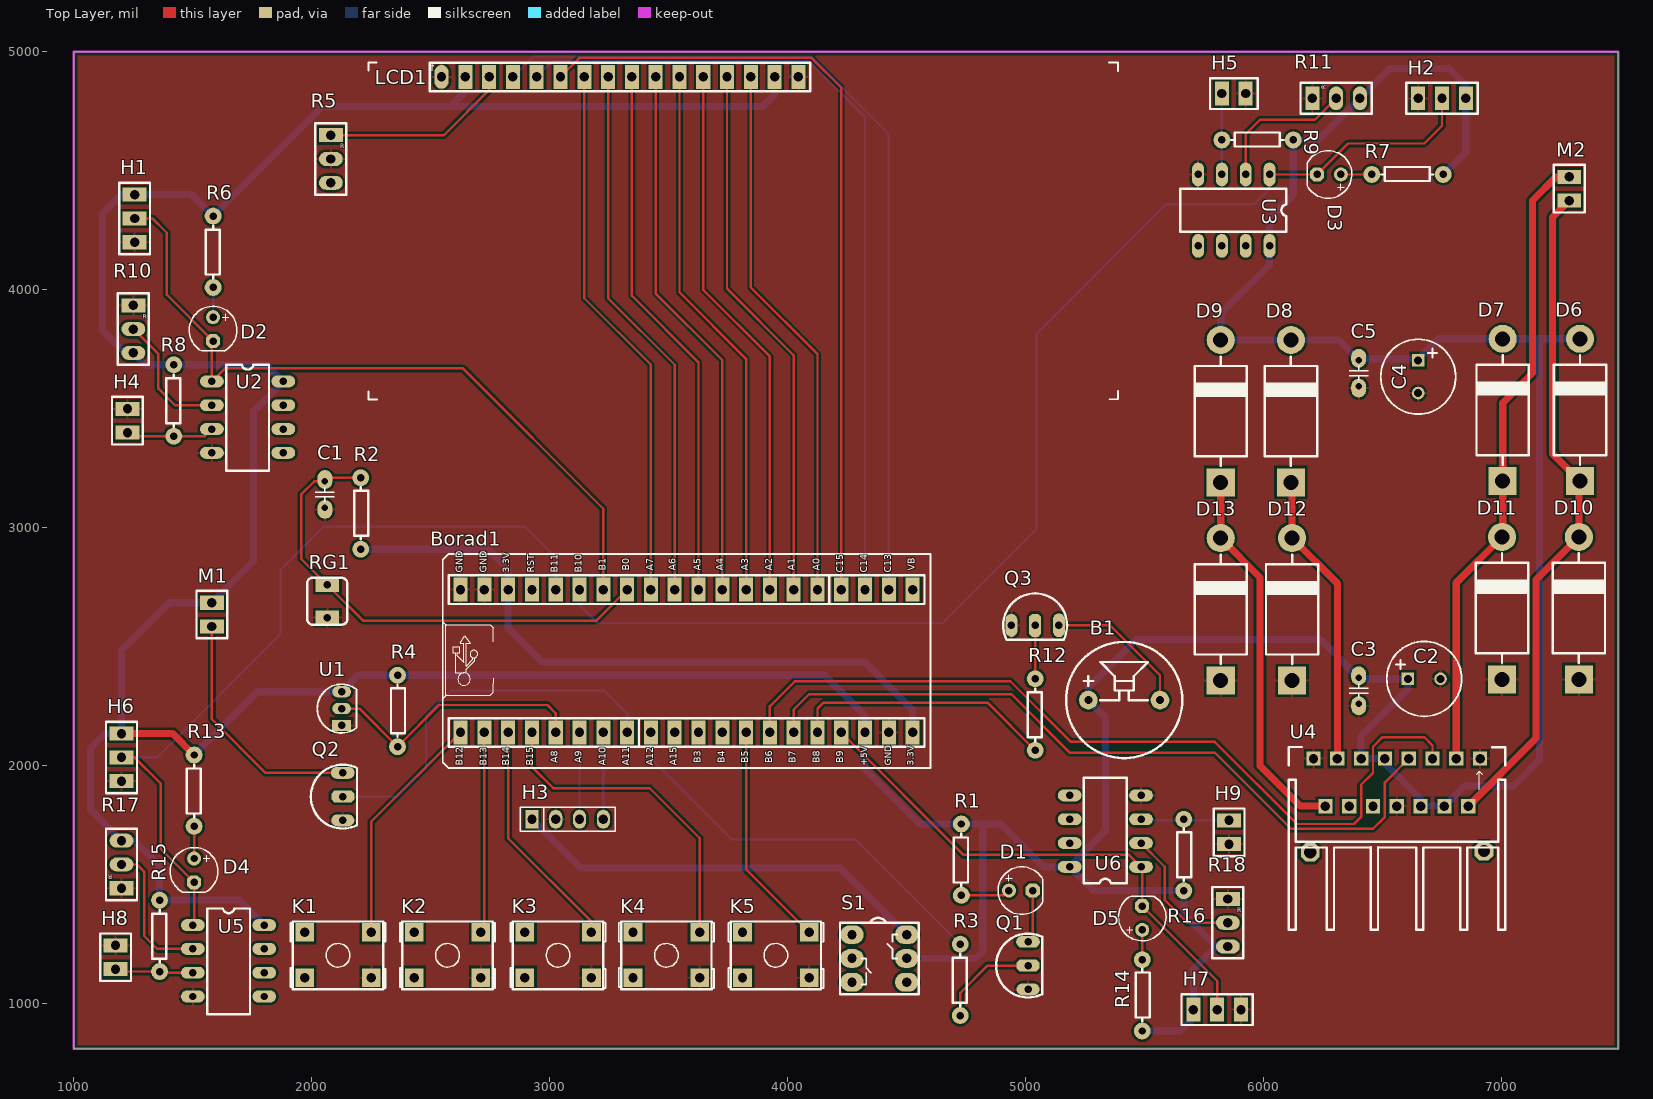
[diagram p0: Top Layer view]
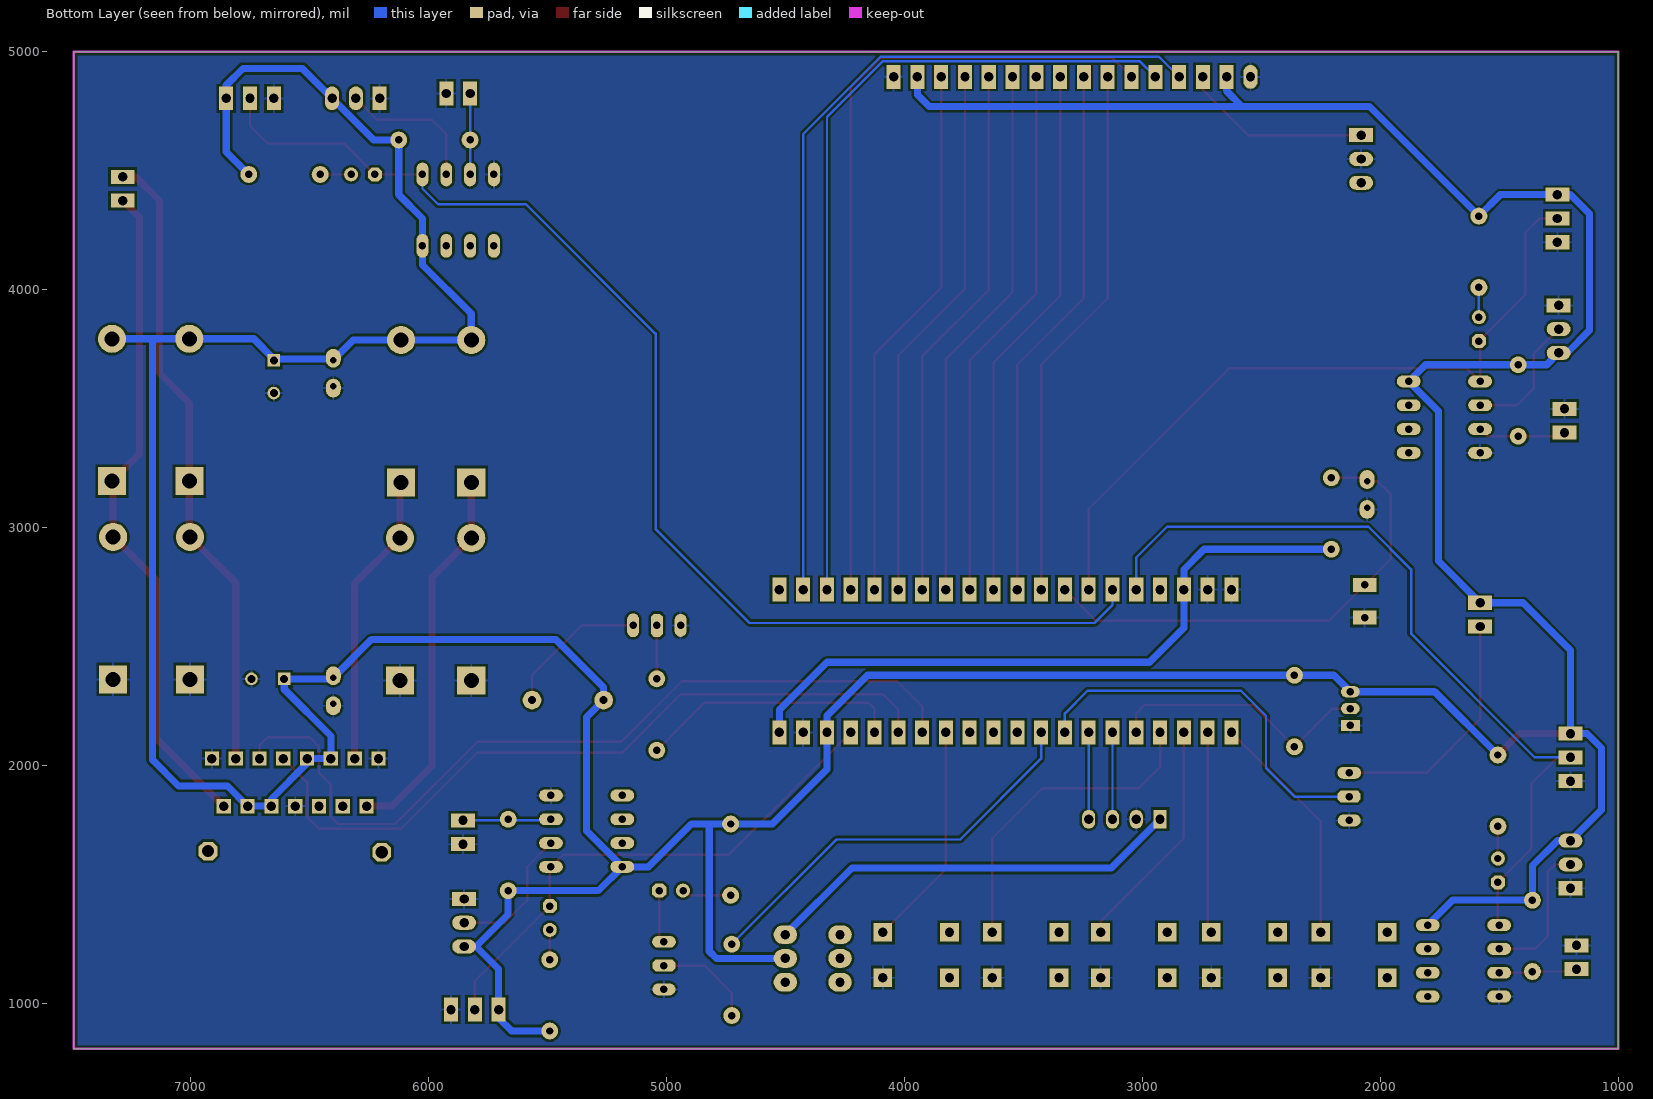
[diagram p1: Bottom Layer view, seen from below]
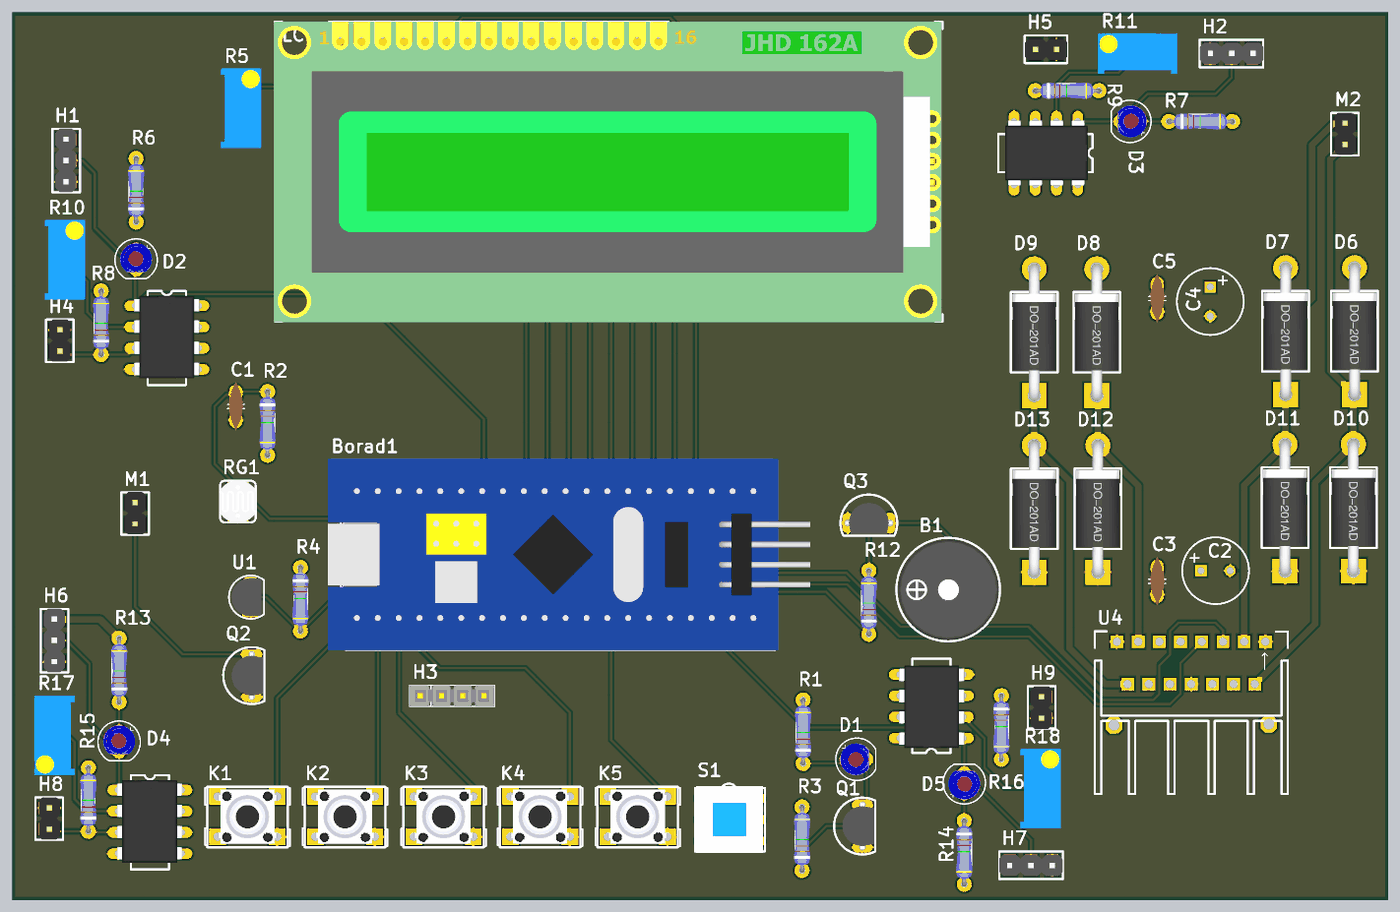
[diagram p2: 3D render of the assembled board from above, using the file's embedded part models]
# Altium PCB MISC82103.PcbDoc
Units mil, origin at the board's own origin, x right, y up, seen from the top; angles counter-clockwise.
Board outline 6490 x 4190 mil, 2 copper layers (Top Layer, Bottom Layer); 66 components, 56 nets, 252 pads, 0 vias.

## Layer stack, top to bottom (the 12.6 mil dielectric is the usual default, probably not edited)
Top Solder: solder mask 0.4, Solder Resist, Dk 3.5
Top Layer: signal copper 1.4
Dielectric 1: dielectric 12.6, FR-4, Dk 4.8
Bottom Layer: signal copper 1.4
Bottom Solder: solder mask 0.4, Solder Resist, Dk 3.5

## Board outline
1000,810 1000,5000 7490,5000 7490,810

## Design rules (kind name [scope] priority, off if disabled: settings)
Clearance [All] p1: gap=10
MinimumSolderMaskSliver [All] p1: minsoldermaskwidth=0
PolygonConnect [All] p1: connectstyle=Relief reliefconductorwidth=10 reliefentries=4 polygonreliefangle="90 Angle" airgapwidth=10
RoutingVias [All] p1: holewidth=28 width=50 viastyle="Through Hole" minholewidth=28 minwidth=50 maxholewidth=28 maxwidth=50
SilkToSilkClearance [All] p1: silktosilkclearance=0
SilkToSolderMaskClearance [IsPad] p1: minsilkscreentomaskgap=0 clearancetoexposedcopper=TRUE
SolderMaskExpansion [All] p1: expansion=4
Width [All] p1: maxlimit=50 minlimit=10 preferedwidth=10
27 further rules are at their usual default settings.

## Components (designator, comment, footprint, x,y, rotation, side; value= is the part's Value field where it differs from the comment)
B1 "Buzzer" BUZZER 5263.51,2275.91 r0 top
Borad1 "STM32F103C6T6_Borad" STM32F103C8T6_买的 2625,2140 r0 top
C1 "0.1uF" "CAP - 2.54mm" 2055,3140 r90 top
C2 "220uF" "CAPe - 3.5MM" 6675,2365 r0 top
C3 "0.1uF" "CAP - 2.54mm" 6400,2315 r90 top
C4 "220uF" "CAPe - 3.5MM" 6650,3635 r270 top
C5 "0.1uF" "CAP - 2.54mm" 6400,3650 r90 top
D1 "LED" LED-3MM 4980,1475 r180 top
D2 "LED" LED-3MM 1585,3835 r90 top
D3 "LED" LED-3MM 6275,4485 r0 top
D4 "LED" LED-3MM 1505,1560 r90 top
D5 "LED" LED-3MM 5490,1360 r270 top
D6 "1N4007" "DIODE - 15.24mm" 7330,3495 r270 top
D7 "1N4007" "DIODE - 15.24mm" 7005,3495 r270 top
D8 "1N4007" "DIODE - 15.24mm" 6115,3490 r270 top
D9 "1N4007" "DIODE - 15.24mm" 5820,3490 r270 top
D10 "1N4007" "DIODE - 15.24mm" 7325,2662.27 r270 top
D11 "1N4007" "DIODE - 15.24mm" 7002.36,2662.27 r270 top
D12 "1N4007" "DIODE - 15.24mm" 6120,2657.27 r270 top
D13 "1N4007" "DIODE - 15.24mm" 5820,2657.27 r270 top
H1 "CON3" CON3 1255,4300 r0 top
H2 "CON3" CON3 6750,4805 r270 top
H3 "Program download interface" CON4 3075,1775 r90 top
H4 "CON2" CON2 1225,3500 r0 top
H5 "CON2" CON2 5925,4825 r270 top
H6 "CON3" CON3 1200,2035 r0 top
H7 "CON3" CON3 5805,975 r90 top
H8 "CON2" CON2 1175,1245 r0 top
H9 "CON2" CON2 5855,1670 r180 top
K1 "Key" Buttom 2110,1205 r180 top
K2 "Key" Buttom 2570,1205 r180 top
K3 "Key" Buttom 3035,1205 r180 top
K4 "Key" Buttom 3490,1205 r180 top
K5 "Key" Buttom 3950,1205 r180 top
LCD1 "LCD1602" LCD1602 2545,4895 r0 top
M1 "FAN" CON2 1580,2685 r0 top
M2 "MOTTOR" CON2 7285,4475 r0 top
Q1 "NPN" "NPN & PNP" 5010,1160 r0 top
Q2 "NPN" "NPN & PNP" 2130,1870 r0 top
Q3 "NPN" "NPN & PNP" 5040,2590 r270 top
R1 "330R" Resistor-7.62mm 4730,1455 r90 top
R2 "10K" Resistor-7.62mm 2205,3210 r270 top
R3 "1K" Resistor-7.62mm 4725,950 r90 top
R4 "10K" Resistor-7.62mm 2360,2380 r270 top
R5 "10K" Res_Variable-DIP 2080,4650 r0 top
R6 "300R" Resistor-7.62mm 1585,4010 r90 top
R7 "300R" Resistor-7.62mm 6455,4485 r0 top
R8 "1M" Resistor-7.62mm 1420,3385 r90 top
R9 "1M" Resistor-7.62mm 5825,4630 r0 top
R10 "10K" Res_Variable-DIP 1250,3935 r0 top
R11 "10K" Res_Variable-DIP 6205,4805 r90 top
R12 "1K" Resistor-7.62mm 5040,2065 r90 top
R13 "300R" Resistor-7.62mm 1505,1745 r90 top
R14 "300R" Resistor-7.62mm 5490,1185 r270 top
R15 "1M" Resistor-7.62mm 1360,1135 r90 top
R16 "1M" Resistor-7.62mm 5665,1775 r270 top
R17 "10K" Res_Variable-DIP 1200,1485 r180 top
R18 "10K" Res_Variable-DIP 5850,1440 r0 top
RG1 "1M" RG 2065,2622.2 r180 top
S1 "Latching switch" Switch 4270,1190 r0 top
U1 "DS18B20" DS18B20 2125,2240 r90 top
U2 "LM358" DIP8 1780,3415 r0 top
U3 "LM358" DIP8 5825,4285 r270 top
U4 "L298N-DIP" L298N 6561,1931 r180 top
U5 "LM358" DIP8 1700,1130 r0 top
U6 "LM358" DIP8 5285,1775 r180 top

## Footprints (in the part's own frame and the unit in brackets; to place one, negate y for a bottom-side part, rotate by r counter-clockwise, add the part's x,y. Pads: shape width x height; smd on the part's side, far side on the other; paste and mask are expansions set on the pad)
Buttom [mm]
  rect 2x2 hole 1: 1(-3.556,2.438) 2(-3.556,-2.413) 3(3.556,-2.413) 4(3.556,2.438)
  silkscreen extent -5.08,-3.56 5.08,3.68, body extent -4.13,-3.22 4.13,3.28, height 5
BUZZER [mm] "蜂鸣器-DIP直插封装"
  round 2 hole 0.85: 1(0,0) 2(7.65,0)
  silkscreen extent -2.38,-6.2 10.02,6.2, body extent -2.14,-6.03 9.86,5.97, height 9.3
"CAP - 2.54mm" [mm] "2.54mm脚距陶瓷电容"
  oval 2x1.6 hole 0.7 copper offset -0.2,0: 1(-1.397,0)
  oval 2x1.6 hole 0.7 copper offset 0.2,0: 2(1.397,0)
  silkscreen extent -0.76,-1.02 0.76,1.02, body extent -2.9,-0.85 2.94,0.85, height 5.92
"CAPe - 3.5MM" [mm]
  rect 1.35x1.35 hole 0.85: 1(-1.75,0)
  round 1.35 hole 0.85: 2(1.75,0)
  silkscreen extent -4,-4 4,4
CON2 [mm]
  rect 2.54x1.5 hole 1: 1(0,0) 2(0,-2.54)
  silkscreen extent -1.65,-3.81 1.65,1.27, body extent -1.24,-3.78 1.3,1.3, height 8.54
CON3 [mm]
  rect 2.54x1.5 hole 1: 1(0,2.54) 2(0,0) 3(0,-2.54)
  silkscreen extent -1.65,-3.81 1.65,3.81, body extent -1.3,-3.78 1.24,3.84, height 8.54
CON4 [mm]
  rect 2x1.4 hole 1: 1(0,3.81)
  oval 2x1.4 hole 1: 2(0,1.27) 3(0,-1.27) 4(0,-3.81)
  silkscreen extent -1.27,-5.08 1.27,5.08, body extent -1.27,-5.08 1.27,5.08, height 8.89
"DIODE - 15.24mm" [mm] "间距15.24mm"
  rect 3x3 hole 1.6: 1(7.6,0)
  round 3 hole 1.6: 2(-7.6,0)
  silkscreen extent -5.84,-2.79 5.84,2.79, body extent -8.25,-2.6 8.25,2.6, height 5.25
DIP8 [mm]
  oval 2.54x1.27 hole 0.8: 1(-5.08,5.08) 2(-5.08,2.54) 3(-5.08,0) 4(-5.08,-2.54) 5(2.54,-2.54) 6(2.54,0) 7(2.54,2.54) 8(2.54,5.08)
  silkscreen extent -3.56,-4.44 1.02,6.85, body extent -5.21,-3.63 2.61,6.28, height 4.57
DS18B20 [mm]
  rect 1.2x2 hole 0.8: 1(-1.8,0)
  oval 1.2x2 hole 0.8: 2(0,0) 3(1.8,0)
  silkscreen extent -2.6,-1.6 2.6,2.6, body extent -2.3,-1.3 2.3,2.3, height 7.6
L298N [mil]
  oct 78.74x78.74 hole 51.18: 0(-365,290) 0(365,295)
  rect 60x60 hole 39.37: 1(-349,-99) 2(-299,101) 3(-249,-99) 4(-199,101) 5(-149,-99) 6(-99,101) 7(-49,-99) 8(1,101) 9(51,-99) 10(101,101) 11(151,-99) 12(201,101) 13(251,-99) 14(301,101) 15(351,-99)
  silkscreen extent -455,-148 455,620
LCD1602 [mm]
  oval 1.5x2.54 hole 1: 1(0,0)
  rect 1.5x2.54 hole 1: 2(2.54,0) 3(5.08,0) 4(7.62,0) 5(10.16,0) 6(12.7,0) 7(15.24,0) 8(17.78,0) 9(20.32,0) 10(22.86,0) 11(25.4,0) 12(27.94,0) 13(30.48,0) 14(33.02,0) 15(35.56,0) 16(38.1,0)
  silkscreen extent -7.8,-34.44 72.21,1.55, body extent -7.92,-34.46 72.08,1.54, height 10.6
LED-3MM [mm]
  oct 1.5x1.5 hole 0.8: 1(-1.27,0)
  round 1.5 hole 0.8: 2(1.27,0)
  silkscreen extent -2.35,-2.54 2.44,2.54, body extent -1.57,-1.9 1.93,1.93, height 5.5
"NPN & PNP" [mm]
  oct 2.45x1.27 hole 0.8: 1(0,0)
  oval 2.45x1.27 hole 0.8: 2(0,-2.54)
  oval 2.54x1.27 hole 0.8: 3(0,2.54)
  silkscreen extent -3.41,-3.41 1.52,3.41, body extent -2.41,-2.84 1.39,2.84, height 6.83
Res_Variable-DIP [mm]
  rect 2.54x1.5 hole 1: 1(0,0)
  oval 2.54x1.5 hole 1: 2(0,-2.54) 3(0,-5.08)
  silkscreen extent -1.65,-6.35 1.65,1.27, body extent -2.42,-7.38 2.41,2.15, height 11.55
Resistor-7.62mm [mm]
  round 1.8 hole 0.8: 1(0,0) 2(7.62,0)
  silkscreen extent 0.98,-0.7 6.58,0.8, body extent -0.25,-0.98 7.87,0.97, height 2.51
RG [mm] "光敏电阻"
  rect 2.54x1.5 hole 0.8: 1(0,0) 2(0,-3.5)
  silkscreen extent -2.13,-4.25 2.13,0.75, body extent -2.15,-4.28 2.15,0.77, height 2.2
STM32F103C8T6_买的 [mm] "买的小系统"
  rect 1.5x2.54 hole 1: 1(0,0) 2(2.54,0) 3(5.08,0) 4(7.62,0) 5(10.16,0) 6(12.7,0) 7(15.24,0) 8(17.78,0) 9(20.32,0) 10(22.86,0) 11(25.4,0) 12(27.94,0) 13(30.48,0) 14(33.02,0) 15(35.56,0) 16(38.1,0) 17(40.64,0) 18(43.18,0) 19(45.72,0) 20(48.26,0) 21(48.26,15.24) 22(45.72,15.24) 23(43.18,15.24) 24(40.64,15.24) 25(38.1,15.24) 26(35.56,15.24) 27(33.02,15.24) 28(30.48,15.24) 29(27.94,15.24) 30(25.4,15.24) 31(22.86,15.24) 32(20.32,15.24) 33(17.78,15.24) 34(15.24,15.24) 35(12.7,15.24) 36(10.16,15.24) 37(7.62,15.24) 38(5.08,15.24) 39(2.54,15.24) 40(0,15.24)
  silkscreen extent -1.91,-3.81 50.16,19.05, body extent -3.48,-3.85 54.32,19.15, height 11.4
Switch [mm]
  oval 2.5x2 hole 1: 1(0,2.54) 2(0,0) 3(0,-2.54) 4(5.842,-2.54) 5(5.842,0) 6(5.842,2.54)
  silkscreen extent -1.27,-3.81 7.11,4.32, body extent -1.12,-3.99 6.88,4.01, height 13.5

## Part data
Borad1: "Core board (purchased online)"
C1 C3 C5: library part CAP, "Non-polar capacitor"
C2 C4: library part CAP-E, "Polar capacitor"
D1: library part LED-RED
D2 D3 D4 D5: library part LED-GREEN
D6 D7 D8 D9 D10 D11 D12 D13: library part Diode, "Rectifier diode / single-direction diode"
H1 H2 H4 H5 H6 H7 H8 H9: "Pin header / terminal block / connector"
H3: library part CON4, "Pin header / terminal block / connector"
K1 K2 K3 K4 K5: "Push button"
M1: "Small fan"
M2: "DC motor"
Q1 Q2 Q3: "NPN transistor"
R1 R2 R3 R4 R6 R7 R8 R9 R12 R13 R14 R15 R16: library part Res, "Resistor"
R5 R10 R11 R17 R18: library part Res_Variable, "Adjustable resistor"
RG1: library part RG, "Photoresistor"
S1: library part Switch, "8*8 power switch / latching switch"
U1: "Temperature sensor"
U2 U3 U5 U6: "Dual operational amplifier"
U4: "Dual H-bridge driver IC"

## Nets (pads, with @x,y where several pads share a name; then routed paths per layer and width w, separated by ;. In a path a pad name is that pad's centre, name@x,y a point inside that pad or via, vN(x,y) a via of type N, cw(c..) or ccw(c..) an arc to the next point about the centre after c; other vN are vias at no path point)
+3.3V: Borad1.20 Borad1.38 R2.2 | length 2838.1
  Bottom Layer w30: R2.2 2740,2910 2825,2825 Borad1.38 2825,2580 2970,2435 4325,2435 4525,2235 Borad1.20
+5V: H3.1 S1.6 | length 1775.9
  Bottom Layer w30: H3.1 3130,1570 4220,1570 S1.6
BUZZER: Borad1.16 R12.1 | length 1108.2
  Top Layer w10: Borad1.16 4125,2240 4150,2265 4840,2265 R12.1
D0: Borad1.32 LCD1.7 | length 2271
  Top Layer w10: LCD1.7 3145,3965 3425,3685 Borad1.32
D1: Borad1.31 LCD1.8 | length 2271
  Top Layer w10: LCD1.8 3245,3965 3525,3685 Borad1.31
D2: Borad1.30 LCD1.9 | length 2271
  Top Layer w10: LCD1.9 3345,3975 3625,3695 Borad1.30
D3: Borad1.29 LCD1.10 | length 2271
  Top Layer w10: LCD1.10 3445,3985 3725,3705 Borad1.29
D4: Borad1.28 LCD1.11 | length 2271
  Top Layer w10: LCD1.11 3545,3990 3825,3710 Borad1.28
D5: Borad1.27 LCD1.12 | length 2271
  Top Layer w10: LCD1.12 3645,4000 3925,3720 Borad1.27
D6: Borad1.26 LCD1.13 | length 2271
  Top Layer w10: LCD1.13 3745,4005 4025,3725 Borad1.26
D7: Borad1.25 LCD1.14 | length 2271
  Top Layer w10: LCD1.14 3845,4010 4125,3730 Borad1.25
DS18B20: Borad1.5 R4.2 U1.2 | length 1133.3
  Top Layer w10: U1.2 2200,2240 R4.2 2535,2255 2990,2255 3025,2220 Borad1.5
EN: Borad1.24 LCD1.6 | length 3375.3
  Top Layer w10: LCD1.6 3045,4895.74 3124.26,4975 4100,4975 4225,4850 Borad1.24
ENA: B1.1 Borad1.18 C2.1 C3.2 C4.1 C5.2 D6.2 D7.2 D8.2 D9.2 H1.1 H2.1 H6.1 H7.1 LCD1.2 LCD1.15 M1.1 R1.2 R4.1 R6.2 R7.2 R8.2 R9.2 R10.3 R11.3 R13.2 R14.2 R15.2 R16.2 R17.3 R18.3 S1.5 U1.3 U2.8 U3.8 U4.4 U4.6 U4.9 U4.11 U5.8 U6.8 | length 24220
  Top Layer w30: H6.1 1415,2135 R13.2
  Bottom Layer w30: R13.2 1770.87,2310.87 U1.3 2194.13,2380 R4.1 4155,2380 4325,2210 Borad1.18 4325,1985 4555,1755 R1.2 4815,1755 ; U5.8 1695,1435 R15.2 1360,1580 1255,1685 R17.3 1070,1815 1070,2075 1130,2135 H6.1 1200,2485 1400,2685 M1.1 1755,2860 1755,3490 U2.8 1810,3685 R8.2 1300,3685 R10.3 1215,3735 1120,3830 1120,4320 1200,4400 H1.1 1495,4400 R6.2 2045,4770 2580,4770 ; LCD1.2 2645,4835 2580,4770 ; LCD1.15 3945,4820 3895,4770 2580,4770 ; S1.5 4500,1189.57 4789.57,1189.57 4820,1220 4820,1750 4815,1755 ; R14.2 5650,885 5705,940 H7.1 5705,1145 R18.3@5800,1240 ; R18.3 R18.3@5800,1240 ; R7.2 6850,4580 H2.1 6850,4860 6780,4930 6530,4930 R11.3 6230,4630 R9.2 6125,4400 6025,4300 U3.8 6025,4105 5820,3900 D9.2 D8.2 6315.79,3789.21 C5.2 6405,3710 6650,3710 6734.21,3794.21 D7.2 7150,3794.21 ; D6.2 7150,3794.21 ; 4815,1755 4895,1755 5075,1575 U6.8 ; U6.8 5335,1725 5335,2204.41 B1.1 5263.51,2328.51 5465,2530 6240,2530 C3.2 6405,2365 C2.1 6606.1,2321.1 6410,2125 U4.11 U4.9 6510,2010 6660,1860 U4.6 U4.4 6845,1915 7050,1915 7160,2025 7160,3784.21 7150,3794.21 ; U6.8 5285,1475 R16.2 5665,1375 R18.3@5800,1240
FAN: Borad1.8 Q2.1 | length 1627.5
  Bottom Layer w10: Q2.1 2360,1870 2480,1990 2480,2210 2585,2315 3230,2315 3325,2220 Borad1.8
GND: Borad1.19 Borad1.39 Borad1.40 C1.1 C2.2 C3.1 C4.2 C5.1 D10.1 D11.1 D12.1 D13.1 H1.3 H2.3 H3.2 H4.1 H5.1 H6.3 H7.3 H8.1 H9.1 K1.1 K2.1 K3.1 K4.1 K5.1 LCD1.1 LCD1.16 Q1.2 Q2.2 Q3.2 R5.2 R10.1 R11.1 R17.1 R18.1 RG1.1 U1.1 U2.4 U3.4 U4.1 U4.8 U4.15 U5.4 U6.4
IN1: Borad1.14 U4.5 | length 3551.2
  Top Layer w10: Borad1.14 3925,2250 4030,2355 4935,2355 5190,2100 5795,2100 6140,1755 6380,1755 6410,1785 6410,1920 6460,1970 6460,2080 6500,2120 6675,2120 6710,2085 U4.5
IN2: Borad1.15 U4.7 | length 3148.1
  Top Layer w10: Borad1.15 4025,2235 4090,2300 4940,2300 5185,2055 5795,2055 6115,1735 6460,1735 6510,1785 6510,1930 U4.7
KEY1: Borad1.1 K1.2 | length 995.3
  Top Layer w10: K1.2 2250,1765 Borad1.1
KEY2: Borad1.2 K2.2 | length 846.2
  Top Layer w10: K2.2 2725,1315 Borad1.2
KEY3: Borad1.3 K3.2 | length 985
  Top Layer w10: Borad1.3 2825,1695 3175,1345 K3.2
KEY4: Borad1.4 K4.2 | length 1369.3
  Top Layer w10: Borad1.4 2925,1995 3015,1905 3420,1905 3630,1695 K4.2
KEY5: Borad1.13 K5.2 | length 949.8
  Top Layer w10: Borad1.13 3825,1565 K5.2
LED-W: Borad1.9 R3.2 | length 1733.1
  Bottom Layer w10: Borad1.9 3425,2030 3765,1690 4285,1690 R3.2
LIGHT: Borad1.33 C1.2 R2.1 RG1.2 | length 2081
  Top Layer w10: R2.1 2070,3210 C1.2 2010,3195 1955,3140 1955,2870 RG1.2 2215,2610 3195.74,2610 3325,2739.26 Borad1.33
M1: D6.1 D10.2 M2.2 U4.2 | length 2816.3
  Top Layer w30: U4.2 7145,2115 7145,2781.48 D10.2 7325,3190.79 D6.1 7215,3310.79 7215,4305 M2.2
M2: D7.1 D11.2 M2.1 U4.3 | length 2674
  Top Layer w30: U4.3 6810,2769.12 D11.2 7005,2964.12 D7.1 7005,3525 7130,3650 7130,4375 7230,4475 M2.1
M3: D8.1 D12.2 U4.13 | length 1241.6
  Top Layer w30: D8.1 6120,3185.79 D12.2 6310,2766.48 U4.13
M4: D9.1 D13.2 U4.14 | length 1604.5
  Top Layer w30: D9.1 D13.2 5985,2791.48 5985,2000 6155,1830 U4.14
NetB1_2: B1.2 Q3.3 | length 615.9
  Top Layer w10: Q3.3 5355,2590 5564.69,2380.31 B1.2
NetD1_1: D1.1 Q1.3 | length 223.3
  Top Layer w10: Q1.3 5030,1280 D1.1
NetD1_2: D1.2 R1.1 | length 208.3
  Top Layer w10: R1.1 4910,1455 D1.2
NetD2_2: D2.2 R6.1 | length 125
  Bottom Layer w10: D2.2 R6.1
NetD3_2: D3.2 R7.1 | length 130
  Top Layer w10: D3.2 R7.1
NetD4_2: D4.2 R13.1 | length 135
  Top Layer w10: D4.2 R13.1
NetD5_2: D5.2 R14.1 | length 125
  Top Layer w10: R14.1 D5.2
NetH4_2: H4.2 R8.1 U2.3 | length 373.6
  Top Layer w10: H4.2 1240,3385 R8.1 1550,3385 U2.3
NetH5_2: H5.2 R9.1 U3.3 | length 340
  Bottom Layer w10: U3.3 R9.1 H5.2
NetH8_2: H8.2 R15.1 U5.3 | length 331.2
  Top Layer w10: H8.2 1185,1135 R15.1 1365,1130 U5.3
NetH9_2: H9.2 R16.1 U6.3 | length 372.1
  Bottom Layer w10: U6.3 5490,1770 H9.2
NetLCD1_3: LCD1.3 R5.1 | length 798.7
  Top Layer w10: R5.1 2555,4650 2745,4840 LCD1.3
NetM1_2: M1.2 Q2.3 | length 1033.2
  Top Layer w10: M1.2 1580,2195 1805,1970 Q2.3
NetQ1_1: Q1.1 R3.1 | length 427.6
  Top Layer w10: R3.1 4725,1045 4840,1160 Q1.1
NetQ3_1: Q3.1 R12.2 | length 225
  Top Layer w10: R12.2 Q3.1
NetR10_2: R10.2 U2.2 | length 547.5
  Top Layer w10: R10.2 1355,3730 1355,3585 1425,3515 U2.2
NetR11_2: R11.2 U3.2 | length 612.6
  Top Layer w10: U3.2 5925,4655 5985,4715 6215.74,4715 6305,4804.26 R11.2
NetR17_2: R17.2 U5.2 | length 605.2
  Top Layer w10: R17.2 1265,1585 1295,1555 1295,1285 1350,1230 U5.2
NetR18_2: R18.2 U6.2 | length 585.8
  Top Layer w10: U6.2 5585,1575 5585,1435 5680,1340 R18.2
P-YH: Borad1.17 D5.1 H7.2 U6.1 | length 2227
  Top Layer w10: Borad1.17 4225,2139.26 4739.26,1625 5435,1625 U6.1 5490,1570 D5.1 5805,1095 H7.2
P-YQ: Borad1.35 D3.1 H2.2 U3.1 | length 5217.3
  Top Layer w10: U3.1 D3.1 6355,4615 6675,4615 6750,4690 H2.2
  Bottom Layer w10: Borad1.35 3125,2675 3200,2600 4650,2600 5045,2995 5045,3815 5590,4360 5960,4360 6025,4425 U3.1
P-ZH: Borad1.36 D4.1 H6.2 U5.1 | length 3459.4
  Top Layer w10: H6.2 1255,2035 1365,1925 1365,1650 D4.1 1505,1335 U5.1
  Bottom Layer w10: H6.2 1350,2035 1870,2555 1870,2825 2050,3005 2895,3005 3025,2875 Borad1.36 Borad1.36@3025,2720
P-ZQ: Borad1.34 D2.1 H1.2 U2.1 | length 3119.9
  Top Layer w10: H1.2 1330,4300 1390,4240 1390,3980 D2.1 1580,3780 U2.1 1635,3670 2635,3670 3225,3080 Borad1.34
RS: Borad1.22 LCD1.4 | length 3665.3
  Bottom Layer w10: LCD1.4 2845,4895.74 2929.26,4980 4100,4980 4425,4655 Borad1.22
RW: Borad1.23 LCD1.5 | length 3490.7
  Bottom Layer w10: LCD1.5 2945,4895.74 3009.26,4960 4091.72,4960 4325,4726.72 Borad1.23
RXD: Borad1.7 H3.4 | length 365
  Bottom Layer w10: H3.4 Borad1.7
TXD: Borad1.6 H3.3 | length 365
  Bottom Layer w10: H3.3 Borad1.6
pads on no net: Borad1.10 Borad1.11 Borad1.12 Borad1.21 Borad1.37 K1.3 K1.4 K2.3 K2.4 K3.3 K3.4 K4.3 K4.4 K5.3 K5.4 R5.3 S1.1 S1.2 S1.3 S1.4 U2.5 U2.6 U2.7 U3.5 U3.6 U3.7 U4.0 U4.10 U4.12 U5.5 U5.6 U5.7 U6.5 U6.6 U6.7

## Polygon pours and split planes (outlines as drawn)
GND on Bottom Layer "G" (solid, remove dead copper, pour order 0): 305,5320 320,5305 7775,5305 7775,500 7745,470 7660,555 445,555
GND on Top Layer "G" (solid, remove dead copper, pour order 2): 775,595 7630,595 7695,530 7765,600 7765,5240 495,5240 445,5290

## Keep-outs
Keep-Out Layer:
  lines w10: 1000,810 1000,1000 1000,4940 1000,5000 1012.07,5000 6995,5000 7490,5000 7490,810 5470,810 1000,810